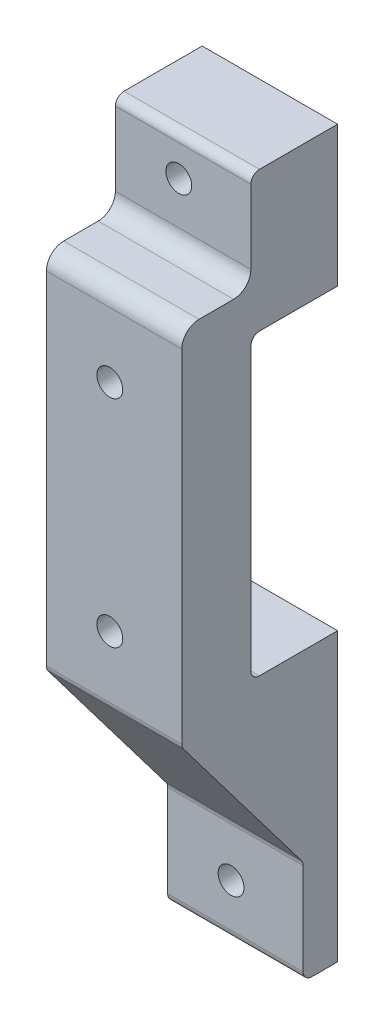
from build123d import *

# Parameters (mm, degrees)
SKETCH1_W            = 16.7
SKETCH1_H            = 40
BOSS_EXTRUDE1_DEPTH  = 2
SKETCH12_W           = 16.7
SKETCH12_H           = 40
BOSS_EXTRUDE4_DEPTH  = 6
SKETCH15_R           = 1.5
CUT_EXTRUDE3_DEPTH   = 24.102434937
SKETCH16_W           = 16.7
SKETCH16_H           = 13.250623967
BOSS_EXTRUDE5_DEPTH  = 6
SKETCH21_W           = 16.7
SKETCH21_H           = 13.250623967
BOSS_EXTRUDE10_DEPTH = 4.06
SKETCH22_W           = 16.7
SKETCH22_H           = 4
BOSS_EXTRUDE11_DEPTH = 20
BOSS_EXTRUDE12_DEPTH = 16.7
SKETCH24_R           = 1.5
CUT_EXTRUDE5_DEPTH   = 54.131010889
SKETCH25_W           = 16.7
SKETCH25_H           = 8
BOSS_EXTRUDE13_DEPTH = 2
FILLET1_R            = 2
FILLET2_R            = 2
SKETCH27_W           = 16.7
SKETCH27_H           = 10.06
BOSS_EXTRUDE14_DEPTH = 3
SKETCH26_R           = 1.5
CUT_EXTRUDE6_DEPTH   = 53.215173256
CUT_EXTRUDE7_DEPTH   = 1
FILLET3_R            = 1


with BuildPart() as part:
    # Sketch1 → Boss-Extrude1 (new body)
    with BuildSketch(Plane.XY):
        Rectangle(SKETCH1_W, SKETCH1_H)
    extrude(amount=BOSS_EXTRUDE1_DEPTH)

    # Sketch12 → Boss-Extrude4 (add)
    with BuildSketch(Plane(origin=(0, 0, 0), x_dir=(-1, 0, 0), z_dir=(0, 0, -1))):
        Rectangle(SKETCH12_W, SKETCH12_H)
    extrude(amount=BOSS_EXTRUDE4_DEPTH)

    # Sketch15 → Cut-Extrude3 (cut, through all)
    with BuildSketch(Plane.XY.offset(2)):
        with Locations((0, 12.5)):
            Circle(SKETCH15_R)
        with Locations((0, -12.5)):
            Circle(SKETCH15_R)
    extrude(amount=-CUT_EXTRUDE3_DEPTH, mode=Mode.SUBTRACT)

    # Sketch16 → Boss-Extrude5 (add)
    with BuildSketch(Plane(origin=(0, 0, -6), x_dir=(-1, 0, 0), z_dir=(0, 0, -1))):
        with Locations((0, 23.926623866)):
            Rectangle(SKETCH16_W, SKETCH16_H)
        with Locations((0, -23.926623866)):
            Rectangle(SKETCH16_W, SKETCH16_H)
    extrude(amount=BOSS_EXTRUDE5_DEPTH)

    # Sketch21 → Boss-Extrude10 (add)
    with BuildSketch(Plane(origin=(0, 0, -12), x_dir=(-1, 0, 0), z_dir=(0, 0, -1))):
        with Locations((0, -23.926623866)):
            Rectangle(SKETCH21_W, SKETCH21_H)
        with Locations((0, 23.926623866)):
            Rectangle(SKETCH21_W, SKETCH21_H)
    extrude(amount=BOSS_EXTRUDE10_DEPTH)

    # Sketch22 → Boss-Extrude11 (add)
    with BuildSketch(Plane.XZ.offset(30.551935849)):
        with Locations((0, -14.06)):
            Rectangle(SKETCH22_W, SKETCH22_H)
    extrude(amount=BOSS_EXTRUDE11_DEPTH)

    # Sketch23 → Boss-Extrude12 (add)
    with BuildSketch(Plane(origin=(8.35, 0, 0), x_dir=(0, 0, -1), z_dir=(1, 0, 0))):
        Polygon((-2, -20), (6, -30.551935849), (12.06, -38.545027255), (12.06, -20), align=None)
    extrude(amount=-BOSS_EXTRUDE12_DEPTH)

    # Sketch24 → Cut-Extrude5 (cut, through all)
    with BuildSketch(Plane.XY.offset(-12.06)):
        with Locations((0, -44.548481552)):
            Circle(SKETCH24_R)
        with Locations((0, 44.548481552)):
            Circle(SKETCH24_R)
    extrude(amount=-CUT_EXTRUDE5_DEPTH, mode=Mode.SUBTRACT)

    # Sketch25 → Boss-Extrude13 (add)
    with BuildSketch(Plane(origin=(0, 20, 0), x_dir=(1, 0, 0), z_dir=(0, 1, 0))):
        with Locations((0, 2)):
            Rectangle(SKETCH25_W, SKETCH25_H)
    extrude(amount=BOSS_EXTRUDE13_DEPTH)

    # Fillet1
    fillet1_edges = [part.edges().sort_by_distance(p)[0] for p in [
        (0, 22, 2),
    ]]
    fillet(fillet1_edges, radius=FILLET1_R)

    # Fillet2
    fillet2_edges = [part.edges().sort_by_distance(p)[0] for p in [
        (0, 22, -6),
    ]]
    fillet(fillet2_edges, radius=FILLET2_R)

    # Sketch27 → Boss-Extrude14 (add)
    with BuildSketch(Plane(origin=(0, 30.551935849, 0), x_dir=(1, 0, 0), z_dir=(0, 1, 0))):
        with Locations((0, 11.03)):
            Rectangle(SKETCH27_W, SKETCH27_H)
    extrude(amount=BOSS_EXTRUDE14_DEPTH)

    # Sketch26 → Cut-Extrude6 (cut, through all)
    with BuildSketch(Plane.XY.offset(-6)):
        with Locations((0, 28.951518448)):
            Circle(SKETCH26_R)
    extrude(amount=-CUT_EXTRUDE6_DEPTH, mode=Mode.SUBTRACT)

    # Sketch28 → Cut-Extrude7 (cut)
    with BuildSketch(Plane.ZY.offset(8.35)):
        with BuildLine():
            Line((2, -20), (2, 20))
            ThreePointArc((2, 20), (1.414213562, 21.414213562), (0, 22))
            Line((0, 22), (-4, 22))
            ThreePointArc((-4, 22), (-5.414213562, 22.585786438), (-6, 24))
            Line((-6, 24), (-6, 33.551935849))
            Line((-6, 33.551935849), (-16.06, 33.551935849))
            Line((-16.06, 33.551935849), (-16.06, 17.301311882))
            Line((-16.06, 17.301311882), (-6, 17.301311882))
            Line((-6, 17.301311882), (-6, -17.301311882))
            Line((-6, -17.301311882), (-16.06, -17.301311882))
            Line((-16.06, -17.301311882), (-16.06, -50.551935849))
            Line((-16.06, -50.551935849), (-12.06, -50.551935849))
            Line((-12.06, -50.551935849), (-12.06, -38.545027255))
            Line((-12.06, -38.545027255), (2, -20))
        make_face()
    extrude(amount=-CUT_EXTRUDE7_DEPTH, mode=Mode.SUBTRACT)

    # Fillet3
    fillet3_edges = [part.edges().sort_by_distance(p)[0] for p in [
        (0.5, 33.551935849, -6),
        (0.5, -20, 2),
        (0.5, -38.545027255, -12.06),
        (0.5, -17.301311882, -6),
        (0.5, 17.301311882, -6),
        (0.5, -50.551935849, -12.06),
    ]]
    fillet(fillet3_edges, radius=FILLET3_R)


solid = part.part
